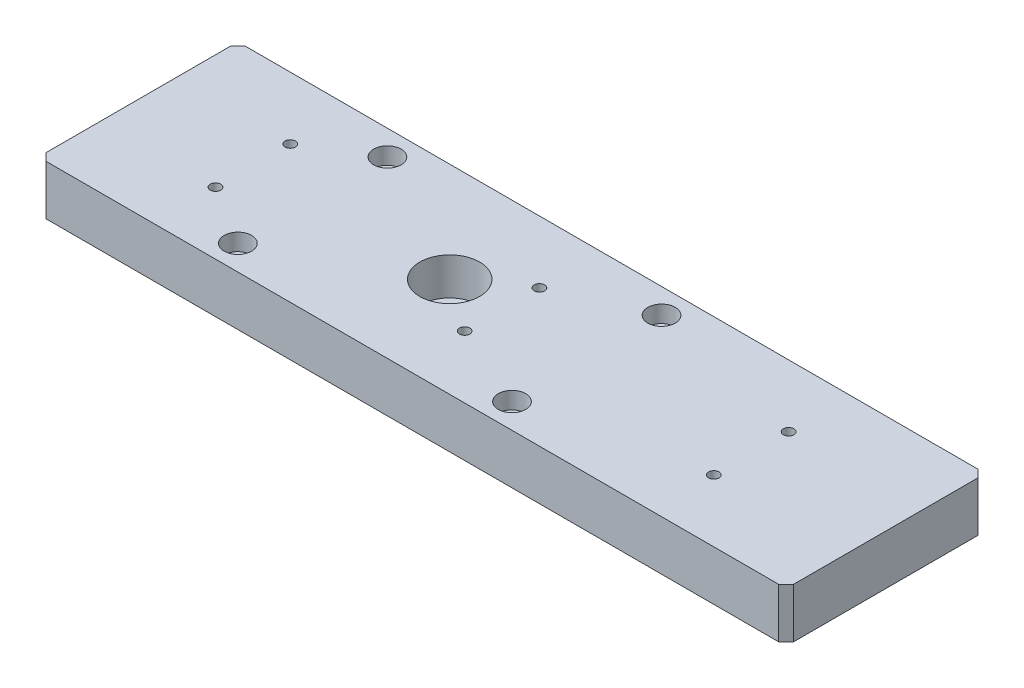
SolidWorks part; units mm, degrees
material "A6061 T6"
ref_plane "前视基准面" through (0, 0, 0) normal (0, 0, 1) x (1, 0, 0)
ref_plane "上视基准面" through (0, 0, 0) normal (0, 1, 0) x (1, 0, 0)
ref_plane "右视基准面" through (0, 0, 0) normal (1, 0, 0) x (0, 0, -1)
sketch "草图1" plane through (0, 0, 0) normal (0, 1, 0) x (1, 0, 0)
  line L1 (-150, 40) -> (150, 40)
  line L2 (-150, 40) -> (-150, -40)
  line L3 (-150, -40) -> (150, -40)
  line L4 (150, 40) -> (150, -40)
  line L5 (-150, 40) -> (150, -40) construction
  line L6 (-150, -40) -> (150, 40) construction
  point P0 (0, 0)
  dimension "D1" = 80
  dimension "D2" = 300
extrude "凸台-拉伸1" add sketch "草图1" along normal blind 20
chamfer "倒角1" distance 3 angle 45 4 edges at (-150, 10, -40) (150, 10, -40) (150, 10, 40) (-150, 10, 40)
hole_wizard "打孔尺寸(%根据)内六角圆柱头螺钉的类型1" positions "草图2" profile "草图3" counterbore size "M14" standard "GB"
sketch "草图2" plane through (0, 20, 0) normal (0, 1, 0) x (1, 0, 0)
  line L0 (-147, -40) -> (147, -40) construction
  line L1 (-150, 37) -> (-150, -37) construction
  point P0 (-25, 0)
  dimension "D1" = 40
  dimension "D2" = 125
sketch "草图3" plane through (-25, 20, 0) normal (1, 0, 0) x (0, 0, 1)
  line L0 (0, 0) -> (0, 29.6567)
  line L1 (0, 29.6567) -> (7.75, 25)
  line L2 (7.75, 25) -> (7.75, 15)
  line L3 (7.75, 15) -> (12, 15)
  line L4 (12, 15) -> (12, 0)
  line L5 (12, 0) -> (0, 0)
  line L10 (0, 29.6567) -> (-7.75, 25) construction
  line L11 (0, -6.35) -> (0, 107.95) construction
  dimension "孔直径" = 15.5
  dimension "孔深度" = 25
  dimension "柱形沉头孔直径" = 24
  dimension "柱形沉头孔深度" = 15
  dimension "导头角度" = 118
hole_wizard "打孔尺寸(%根据)内六角圆柱头螺钉的类型0" positions "草图4" profile "草图5" counterbore size "M6" standard "GB"
sketch "草图4" plane through (0, 20, 0) normal (0, 1, 0) x (1, 0, 0)
  point P0 (30, 30)
  point P2 (-80, 30)
  point P18 (30, -30)
  point P21 (-80, -30)
sketch "草图5" plane through (30, 20, -30) normal (1, 0, 0) x (0, 0, 1)
  line L0 (0, 0) -> (0, 26.9828)
  line L1 (0, 26.9828) -> (3.3, 25)
  line L2 (3.3, 25) -> (3.3, 6.8)
  line L3 (3.3, 6.8) -> (5.5, 6.8)
  line L4 (5.5, 6.8) -> (5.5, 0)
  line L5 (5.5, 0) -> (0, 0)
  line L10 (0, 26.9828) -> (-3.3, 25) construction
  line L11 (0, -6.35) -> (0, 107.95) construction
  dimension "孔直径" = 6.6
  dimension "孔深度" = 25
  dimension "柱形沉头孔直径" = 11
  dimension "柱形沉头孔深度" = 6.8
  dimension "导头角度" = 118
sketch "草图6" plane through (0, 0, 0) normal (0, -1, 0) x (1, 0, 0)
  circle A0 centre (-25, 0) radius 10
  circle A1 centre (30, -30) radius 8.1
  circle A2 centre (-80, -30) radius 8.1
  circle A3 centre (30, 30) radius 8.1
  circle A4 centre (-80, 30) radius 8.1
  dimension "D1" = 20
  dimension "D2" = 16.2
  dimension "D3" = 16.2
  dimension "D4" = 16.2
extrude "切除-拉伸1" cut sketch "草图6" against normal blind 2
hole_wizard "M5 螺纹孔1" positions "草图7" profile "草图8" tap size "M5" standard "GB" end condition through all
sketch "草图7" plane through (0, 0, 0) normal (0, -1, 0) x (-1, 0, 0)
  point P14 (-96, -15)
  point P17 (-96, 15)
  point P20 (4, -15)
  point P23 (4, 15)
  point P26 (104, -15)
  point P29 (104, 15)
cosmetic thread "孔螺蚊线1" parameters "D2"=5
cosmetic thread "孔螺蚊线2" parameters "D2"=5
cosmetic thread "孔螺蚊线3" parameters "D2"=5
cosmetic thread "孔螺蚊线4" parameters "D2"=5
cosmetic thread "孔螺蚊线5" parameters "D2"=5
cosmetic thread "孔螺蚊线6" parameters "D2"=5
sketch "草图8" plane through (96, 0, 15) normal (1, 0, 0) x (0, 0, -1)
  line L0 (0, 0) -> (0, 20)
  line L1 (0, 20) -> (2.1, 20)
  line L2 (2.1, 20) -> (2.1, 0)
  line L5 (2.1, 0) -> (0, 0)
  line L11 (0, -6.35) -> (0, 107.95) construction
  dimension "通孔螺纹孔钻头直径" = 4.2
  dimension "通孔螺纹孔钻头深度" = 20
hole_wizard "M5 螺纹孔2" positions "草图9" profile "草图10" tap size "M5" standard "GB"
sketch "草图9" plane through (0, 0, -40) normal (0, 0, -1) x (-1, 0, 0)
  point P0 (-142, 10)
  point P3 (-130, 10)
sketch "草图10" plane through (142, 10, -40) normal (1, 0, 0) x (0, 1, 0)
  line L0 (0, 0) -> (0, 13.6618)
  line L1 (0, 13.6618) -> (2.1, 12.4)
  line L2 (2.1, 12.4) -> (2.1, 0)
  line L5 (2.1, 0) -> (0, 0)
  line L10 (0, 13.6618) -> (-2.1, 12.4) construction
  line L11 (0, -6.35) -> (0, 107.95) construction
  dimension "螺纹孔钻头直径" = 4.2
  dimension "螺纹孔钻头深度" = 12.4
  dimension "导头角度" = 118
cosmetic thread "孔螺蚊线7" parameters "D1"=10, "D2"=5
cosmetic thread "孔螺蚊线8" parameters "D1"=10, "D2"=5
